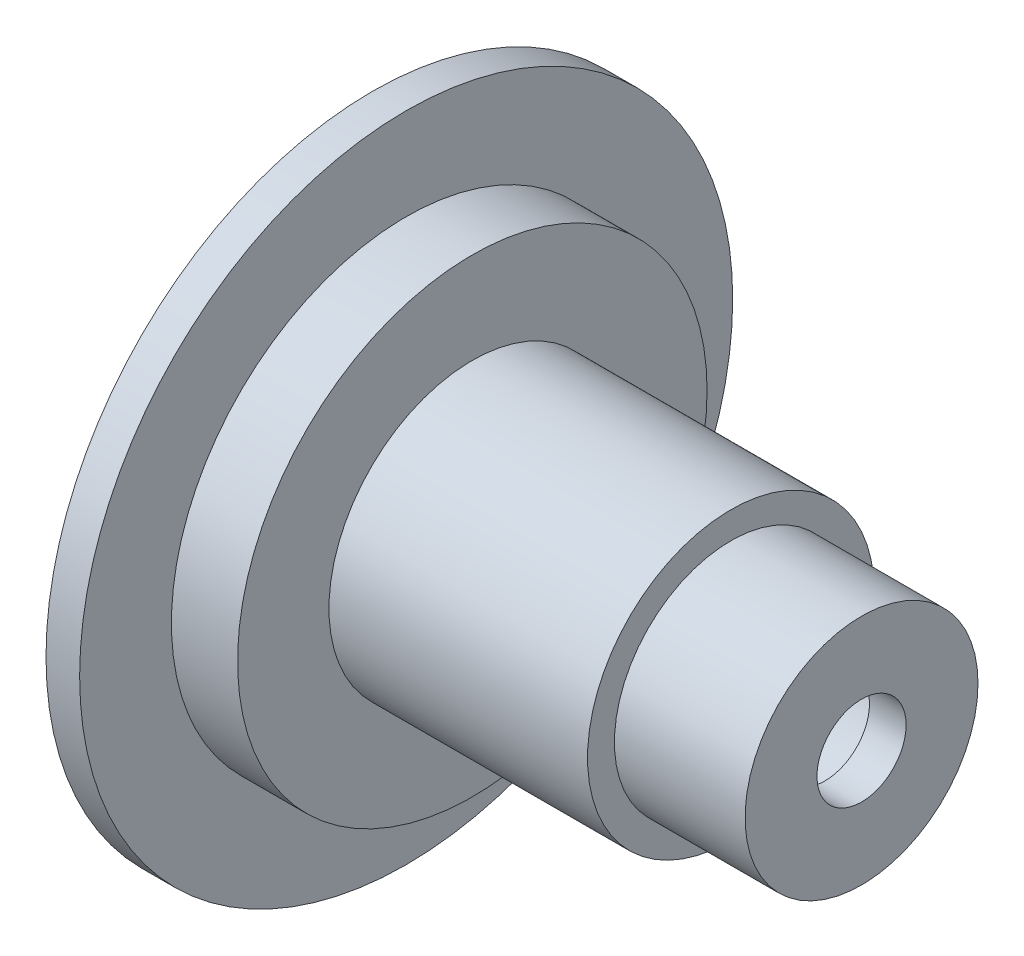
from build123d import *


with BuildPart() as part:
    # Sketch1 → Revolve1 (revolve)
    with BuildSketch(Plane.XY, mode=Mode.PRIVATE) as revolve1_sk:
        Polygon((74.14259961, 24.279053073), (74.14259961, 17.45458405), (79.060819611, 17.45458405), (79.060819611, 10.659632807), (98.286326817, 10.659632807), (98.286326817, 8.659632807), (108, 8.659632807), (108, 3.313609887), (105.27792564, 3.313609887), (105.27792564, 6.159632807), (95.786326817, 6.159632807), (95.786326817, 8.159632807), (76.560819611, 8.159632807), (76.560819611, 14.95458405), (71.64259961, 14.95458405), (71.64259961, 24.279053073), align=None)
    revolve(revolve1_sk.sketch.rotate(Axis((0, 0, 0), (-1, 0, 0)), 90), axis=Axis((0, 0, 0), (-1, 0, 0)))


solid = part.part
